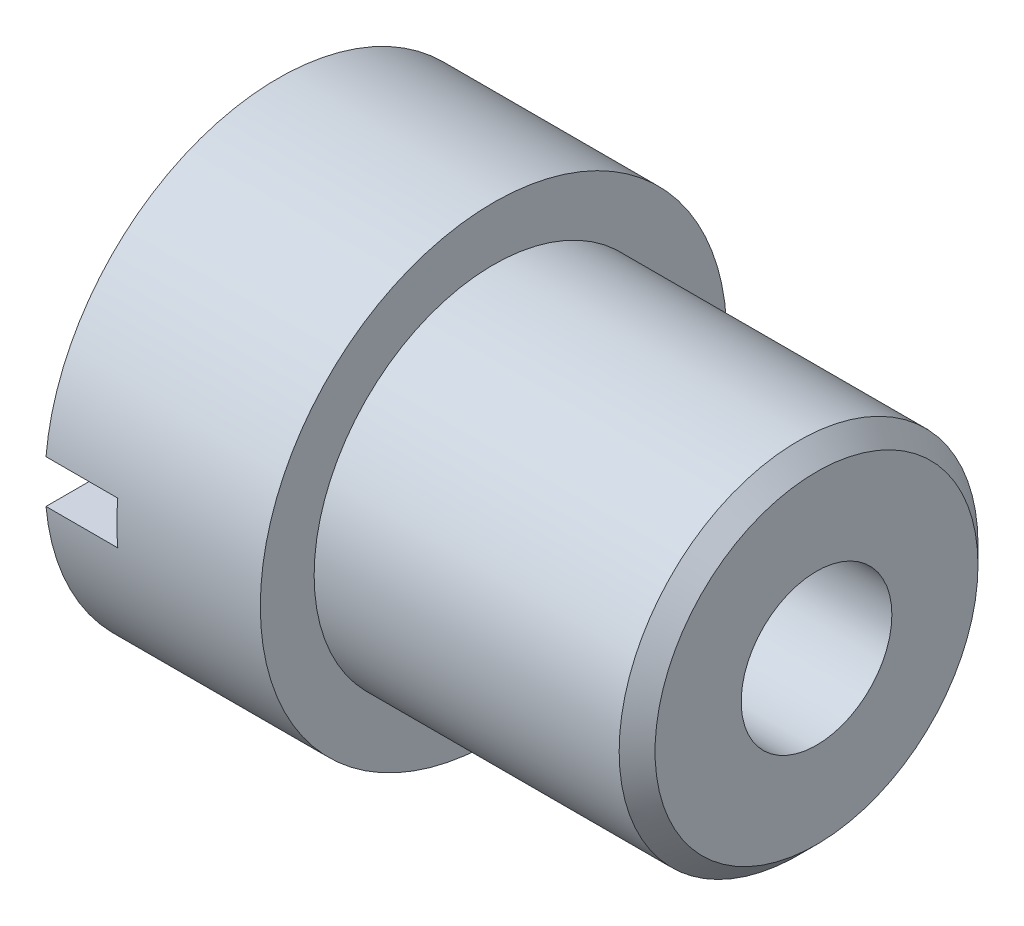
SolidWorks part; units mm, degrees
material "45#"
ref_plane "Front" through (0, 0, 0) normal (0, 0, 1) x (1, 0, 0)
ref_plane "Top" through (0, 0, 0) normal (0, 1, 0) x (1, 0, 0)
ref_plane "Right" through (0, 0, 0) normal (1, 0, 0) x (0, 0, -1)
sketch "草图2" plane through (0, 0, 0) normal (1, 0, 0) x (0, 0, -1)
  circle A0 centre (0, 0) radius 5
  dimension "D1" = 10
extrude "凸台-拉伸1" add sketch "草图2" along normal blind 9
sketch "草图5" plane through (0, 0, 0) normal (-1, 0, 0) x (0, 0, 1)
  circle A0 centre (0, 0) radius 6.5
  dimension "D1" = 13
extrude "凸台-拉伸2" add sketch "草图5" along normal blind 6
sketch "草图6" plane through (-6, 0, 0) normal (-1, 0, 0) x (0, 0, 1)
  line L1 (-15, 0.6) -> (15, 0.6)
  line L2 (-15, 0.6) -> (-15, -0.6)
  line L3 (-15, -0.6) -> (15, -0.6)
  line L4 (15, 0.6) -> (15, -0.6)
  line L5 (-15, 0.6) -> (15, -0.6) construction
  line L6 (-15, -0.6) -> (15, 0.6) construction
  point P0 (0, 0)
  dimension "D1" = 1.2
  dimension "D2" = 30
extrude "切除-拉伸1" cut sketch "草图6" against normal blind 2
hole_wizard "M5 螺纹孔1" positions "3D草图1" profile "草图7" tap size "M5" standard "Gb"
sketch3d "3D草图1"
  line L0 (9, 0, 0) -> (0, 0, 0) construction
  point P0 (9, 0, 0)
sketch "草图7" plane through (9, 0, 0) normal (0, 1, 0) x (0, 0, -1)
  line L0 (0, 0) -> (0, 12.2618)
  line L1 (0, 12.2618) -> (2.1, 11)
  line L2 (2.1, 11) -> (2.1, 0)
  line L5 (2.1, 0) -> (0, 0)
  line L10 (0, 12.2618) -> (-2.1, 11) construction
  line L11 (0, -6.35) -> (0, 107.95) construction
  dimension "螺纹孔钻头直径" = 4.2
  dimension "螺纹孔钻头深度" = 11
  dimension "导头角度" = 118
cosmetic thread "孔螺蚊线1" parameters "D1"=10, "D2"=5
chamfer "倒角1" distance 0.5 angle 45 1 edges at (9, 0, -5)
